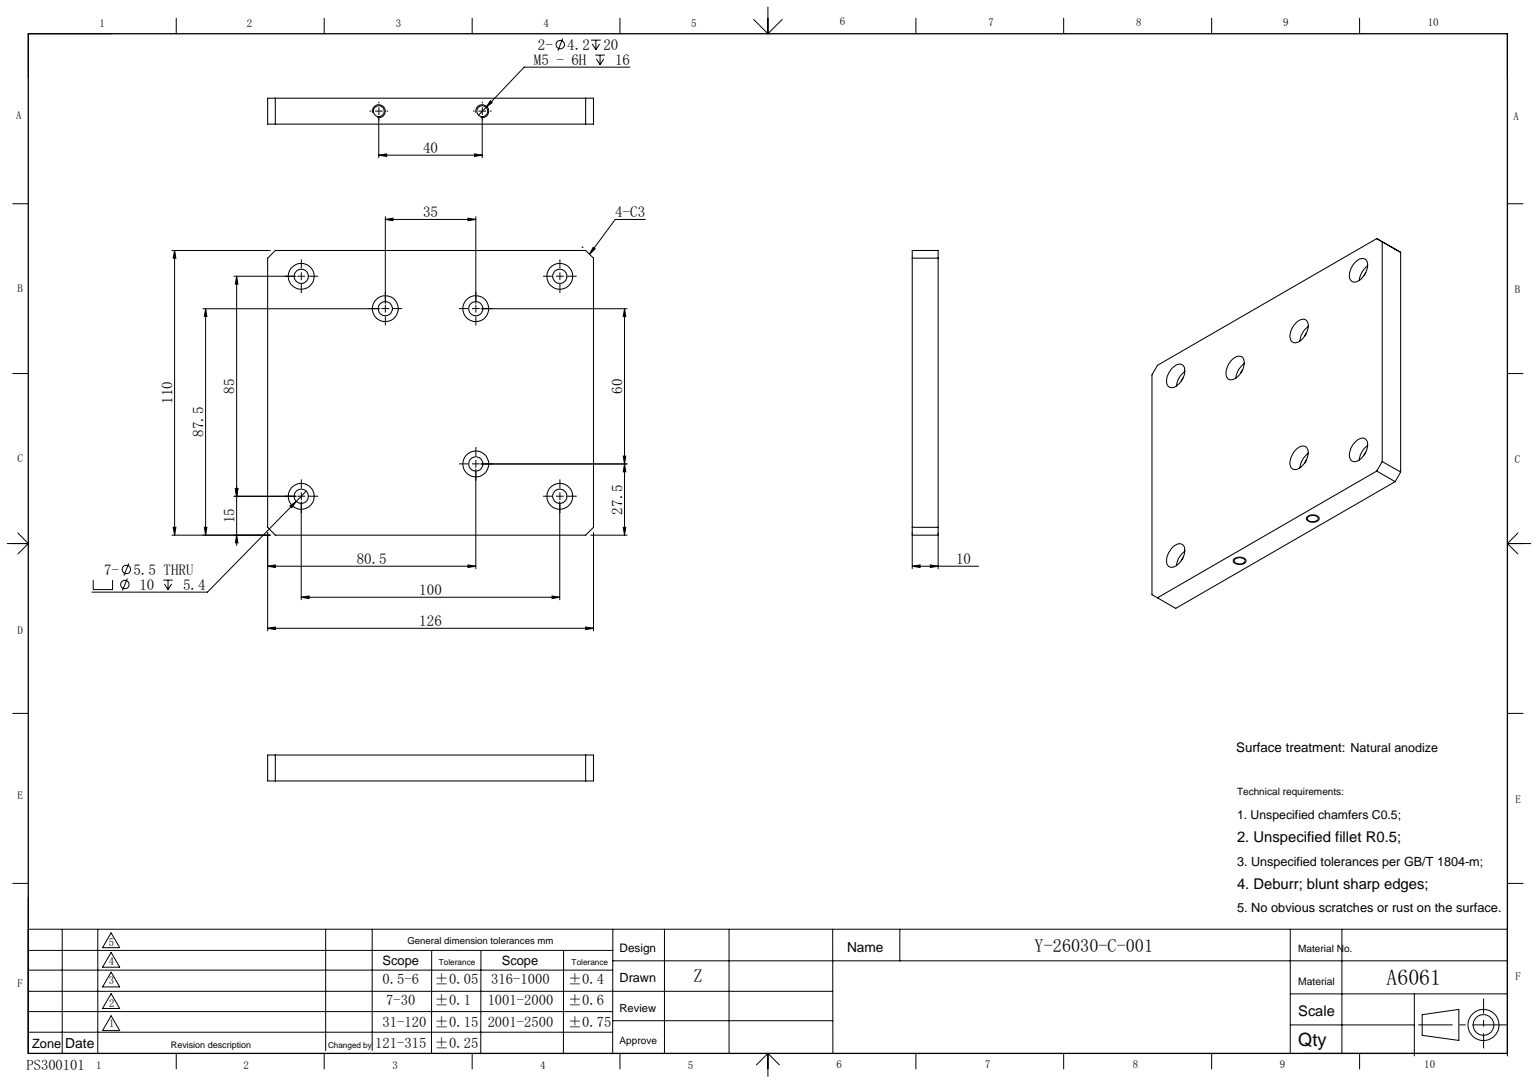
from build123d import *

# Parameters (mm, degrees)
SKETCH_1_W                   = 126
SKETCH_1_H                   = 110
EXTRUDE_1_DEPTH              = 5
CHAMFER_1_SIZE               = 3
HOLE_WIZARD_M5_1_D           = 5.5
HOLE_WIZARD_M5_1_CBORE_D     = 10
HOLE_WIZARD_M5_1_CBORE_DEPTH = 5.4
HOLE_WIZARD_M5_1_2_D         = 4.2
HOLE_WIZARD_M5_1_2_DEPTH     = 20
HOLE_WIZARD_M5_1_2_TIP       = 1.2618073


with BuildPart() as part:
    # 草图1 → 凸台-拉伸1 (new, symmetric)
    with BuildSketch(Plane.XY):
        Rectangle(SKETCH_1_W, SKETCH_1_H)
    extrude(amount=EXTRUDE_1_DEPTH, both=True)

    # 倒角1
    chamfer_1_edges = [part.edges().sort_by_distance(p)[0] for p in [
        (-63, 55, 0),
        (63, 55, 0),
        (63, -55, 0),
        (-63, -55, 0),
    ]]
    chamfer(chamfer_1_edges, length=CHAMFER_1_SIZE)

    # Hole Wizard M5 _1 (through all)
    with Locations(Plane.XY.offset(5)):
        with Locations((-50, 45), (-17.5, 32.5), (17.5, 32.5), (50, 45), (50, -40), (17.5, -27.5), (-50, -40)):
            CounterBoreHole(HOLE_WIZARD_M5_1_D / 2, HOLE_WIZARD_M5_1_CBORE_D / 2, HOLE_WIZARD_M5_1_CBORE_DEPTH)

    # Hole Wizard M5 _1 2
    with Locations(Plane(origin=(0, -55, 0), x_dir=(-1, 0, 0), z_dir=(0, -1, 0))):
        with Locations((20, 0), (-20, 0)):
            Hole(HOLE_WIZARD_M5_1_2_D / 2, depth=HOLE_WIZARD_M5_1_2_DEPTH)
            with Locations((0, 0, -(HOLE_WIZARD_M5_1_2_DEPTH + HOLE_WIZARD_M5_1_2_TIP / 2))):  # 118° drill point
                Cone(0, HOLE_WIZARD_M5_1_2_D / 2, HOLE_WIZARD_M5_1_2_TIP, mode=Mode.SUBTRACT)


solid = part.part
